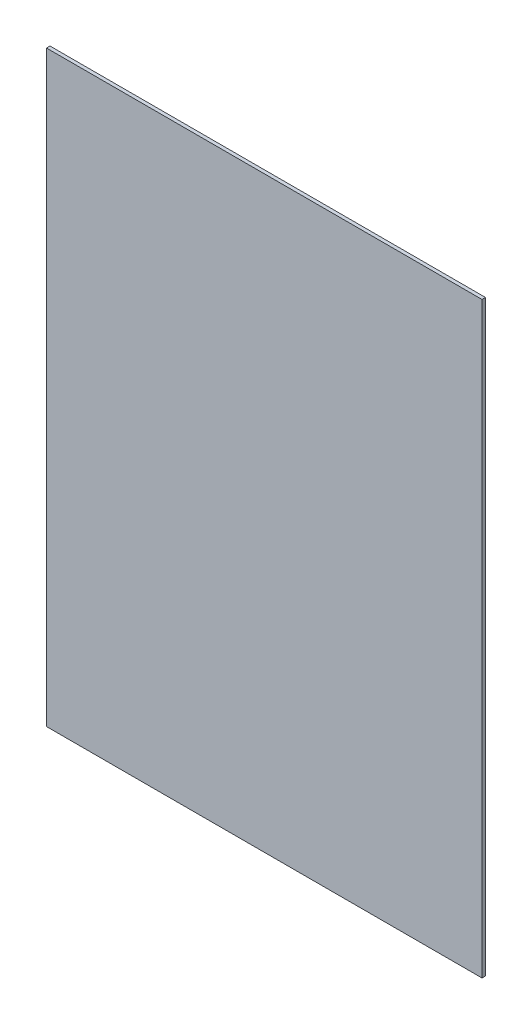
from build123d import *

# Parameters (mm, degrees)
SKETCH_1_W      = 624
SKETCH_1_H      = 842
EXTRUDE_1_DEPTH = 5


with BuildPart() as part:
    # 草图1 → 凸台-拉伸1 (new body)
    with BuildSketch(Plane.XY):
        Rectangle(SKETCH_1_W, SKETCH_1_H)
    extrude(amount=EXTRUDE_1_DEPTH)


solid = part.part
